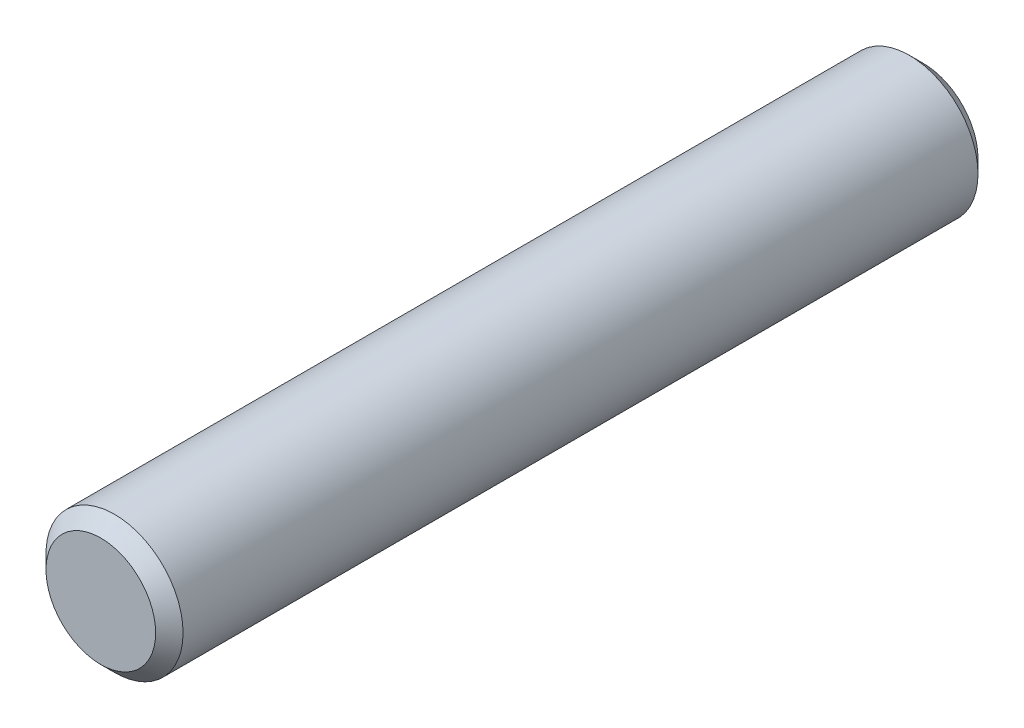
from build123d import *

# Parameters (mm, degrees)
SKETCH1_R           = 2.5
BOSS_EXTRUDE1_DEPTH = 15
CHAMFER1_SIZE       = 0.5


with BuildPart() as part:
    # Sketch1 → Boss-Extrude1 (new, symmetric)
    with BuildSketch(Plane.XY):
        Circle(SKETCH1_R)
    extrude(amount=BOSS_EXTRUDE1_DEPTH, both=True)

    # Chamfer1
    chamfer1_edges = [part.edges().sort_by_distance(p)[0] for p in [
        (-2.5, 0, -15),
        (-2.5, 0, 15),
    ]]
    chamfer(chamfer1_edges, length=CHAMFER1_SIZE)


solid = part.part
